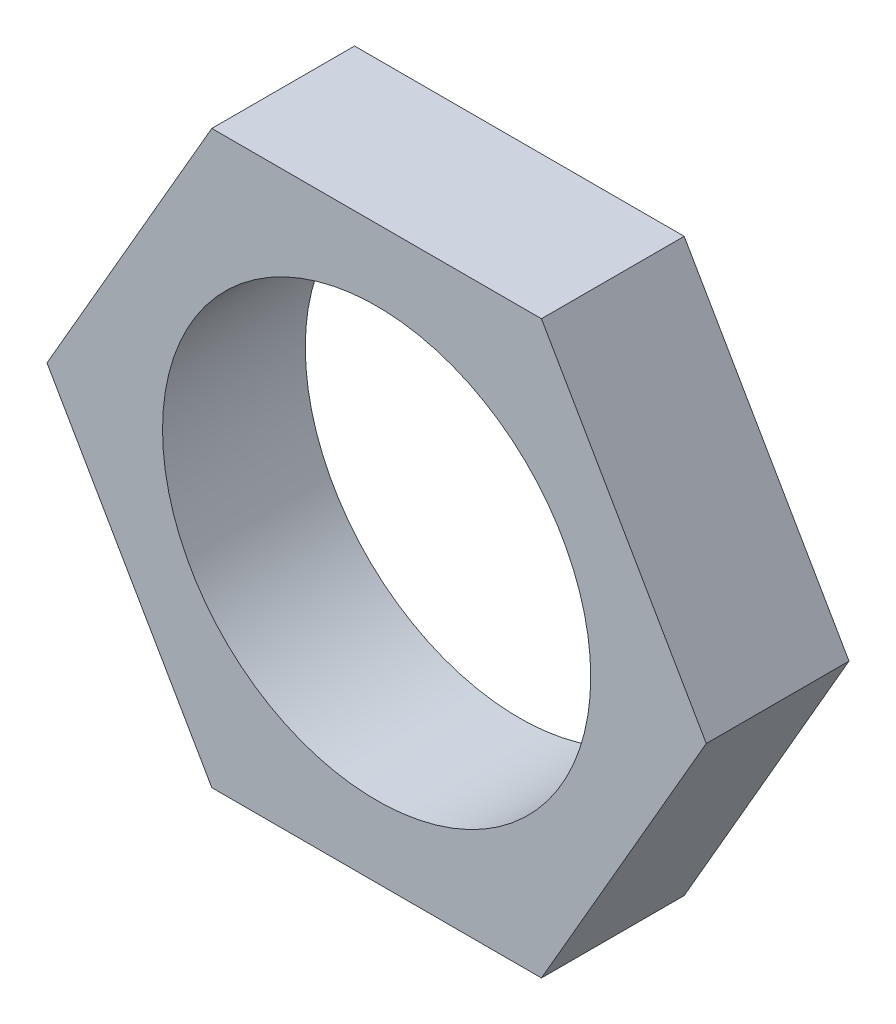
SolidWorks part; units mm, degrees
ref_plane "Front Plane" through (0, 0, 0) normal (0, 0, 1) x (1, 0, 0)
ref_plane "Top Plane" through (0, 0, 0) normal (0, 1, 0) x (1, 0, 0)
ref_plane "Right Plane" through (0, 0, 0) normal (1, 0, 0) x (0, 0, -1)
sketch "Sketch1" plane through (0, 0, 0) normal (0, 0, 1) x (1, 0, 0)
  line L1 (6.9282, 0) -> (3.4641, 6)
  line L2 (3.4641, 6) -> (-3.4641, 6)
  line L3 (-3.4641, 6) -> (-6.9282, 0)
  line L4 (-6.9282, 0) -> (-3.4641, -6)
  line L5 (-3.4641, -6) -> (3.4641, -6)
  line L6 (3.4641, -6) -> (6.9282, 0)
  circle A0 centre (0, 0) radius 6 construction
  dimension "D1" = 12
extrude "Boss-Extrude1" add sketch "Sketch1" along normal blind 3
hole_wizard "M10x1.0 Tapped Hole1" positions "Sketch2" profile "Sketch3" tap size "M10x1.0" standard "GB"
sketch "Sketch2" plane through (0, 0, 3) normal (0, 0, 1) x (1, 0, 0)
  point P0 (0, 0)
sketch "Sketch3" plane through (0, 0, 3) normal (1, 0, 0) x (0, -1, 0)
  line L0 (0, 0) -> (0, 25.7039)
  line L1 (0, 25.7039) -> (4.5, 23)
  line L2 (4.5, 23) -> (4.5, 0)
  line L5 (4.5, 0) -> (0, 0)
  line L10 (0, 25.7039) -> (-4.5, 23) construction
  line L11 (0, -6.35) -> (0, 107.95) construction
  dimension "螺纹孔钻头直径" = 9
  dimension "螺纹孔钻头深度" = 23
  dimension "导头角度" = 118
cosmetic thread "Cosmetic Thread 1"
